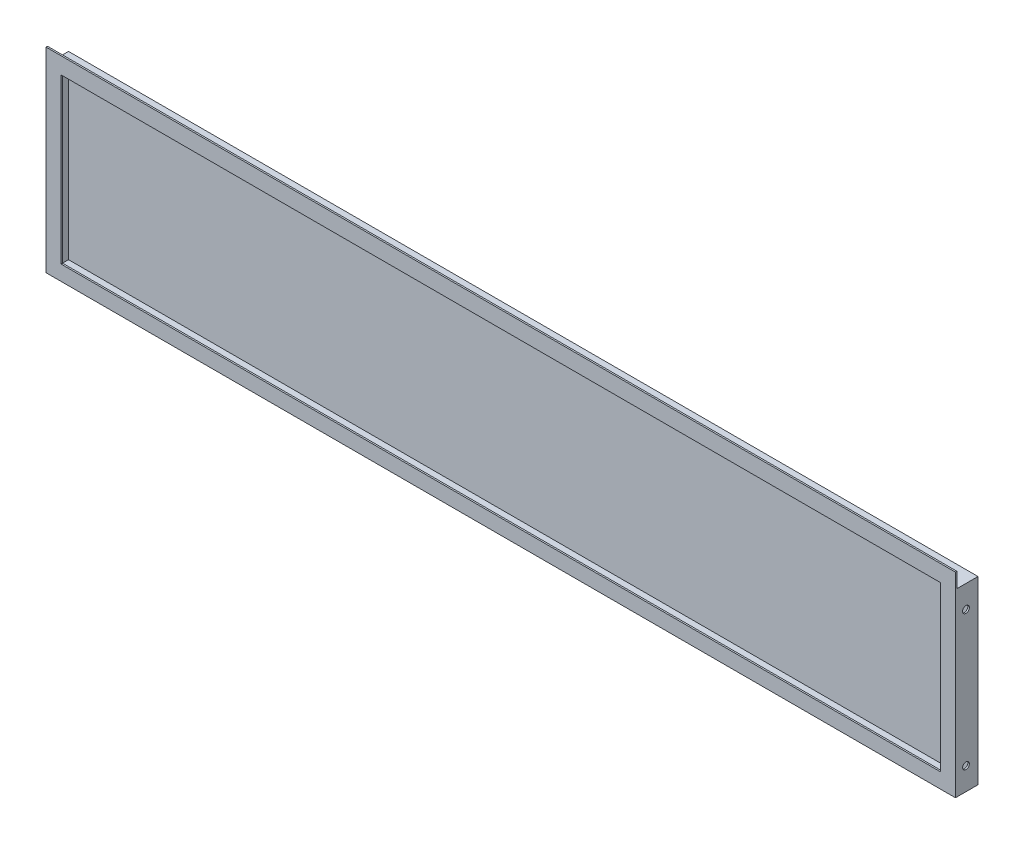
from build123d import *

# Parameters (mm, degrees)
SKETCH_1_W               = 1210
SKETCH_1_H               = 240
EXTRUDE_1_DEPTH          = 30
SHELL_1_T                = -2
SKETCH_2_W               = 1210
SKETCH_2_H               = 260
SKETCH_2_W_2             = 1170
SKETCH_2_H_2             = 218
EXTRUDE_2_DEPTH          = 2
CUT_EXTRUDE_1_DEPTH      = 1316
CUT_EXTRUDE_1_DEPTH_BACK = 198
SKETCH_3_R               = 4.5
SKETCH_4_R               = 4.5
CUT_EXTRUDE_2_DEPTH      = 45


with BuildPart() as part:
    # 草图1 → 凸台-拉伸1 (new body)
    with BuildSketch(Plane.XY):
        with Locations((605, 120)):
            Rectangle(SKETCH_1_W, SKETCH_1_H)
    extrude(amount=EXTRUDE_1_DEPTH)

    # 抽壳1
    shell_1_openings = [part.faces().sort_by_distance(p)[0] for p in [
        (605, 120, 30),
    ]]
    offset(amount=SHELL_1_T, openings=shell_1_openings, kind=Kind.INTERSECTION)

    # 草图2 → 凸台-拉伸2 (add)
    with BuildSketch(Plane.XY.offset(30)):
        with Locations((605, 130)):
            Rectangle(SKETCH_2_W, SKETCH_2_H)
        with Locations((605, 129)):
            Rectangle(SKETCH_2_W_2, SKETCH_2_H_2, mode=Mode.SUBTRACT)
    extrude(amount=-EXTRUDE_2_DEPTH)

    # 草图3 → 切除-拉伸1 (cut, two sides: drawn at the far end of the back side and taken through both)
    with BuildSketch(Plane(origin=(2, 0, 0), x_dir=(0, 0, -1), z_dir=(1, 0, 0)).offset(-CUT_EXTRUDE_1_DEPTH_BACK)):
        with Locations(Location((-16, 30, 0), (0, 0, 180))):
            Circle(SKETCH_3_R)
        with Locations(Location((-16, 210, 0), (0, 0, 180))):
            Circle(SKETCH_3_R)
    extrude(amount=CUT_EXTRUDE_1_DEPTH + CUT_EXTRUDE_1_DEPTH_BACK, mode=Mode.SUBTRACT)

    # 草图4 → 切除-拉伸2 (cut)
    with BuildSketch(Plane(origin=(0, 2, 0), x_dir=(1, 0, 0), z_dir=(0, 1, 0))):
        with Locations(Location((30, -16, 0), (0, 0, 270))):
            Circle(SKETCH_4_R)
        with Locations(Location((1180, -16, 0), (0, 0, 270))):
            Circle(SKETCH_4_R)
        with Locations(Location((680, -16, 0), (0, 0, 270))):
            Circle(SKETCH_4_R)
        with Locations(Location((320, -16, 0), (0, 0, 270))):
            Circle(SKETCH_4_R)
        with Locations(Location((740, -16, 0), (0, 0, 270))):
            Circle(SKETCH_4_R)
    extrude(amount=-CUT_EXTRUDE_2_DEPTH, mode=Mode.SUBTRACT)


solid = part.part
